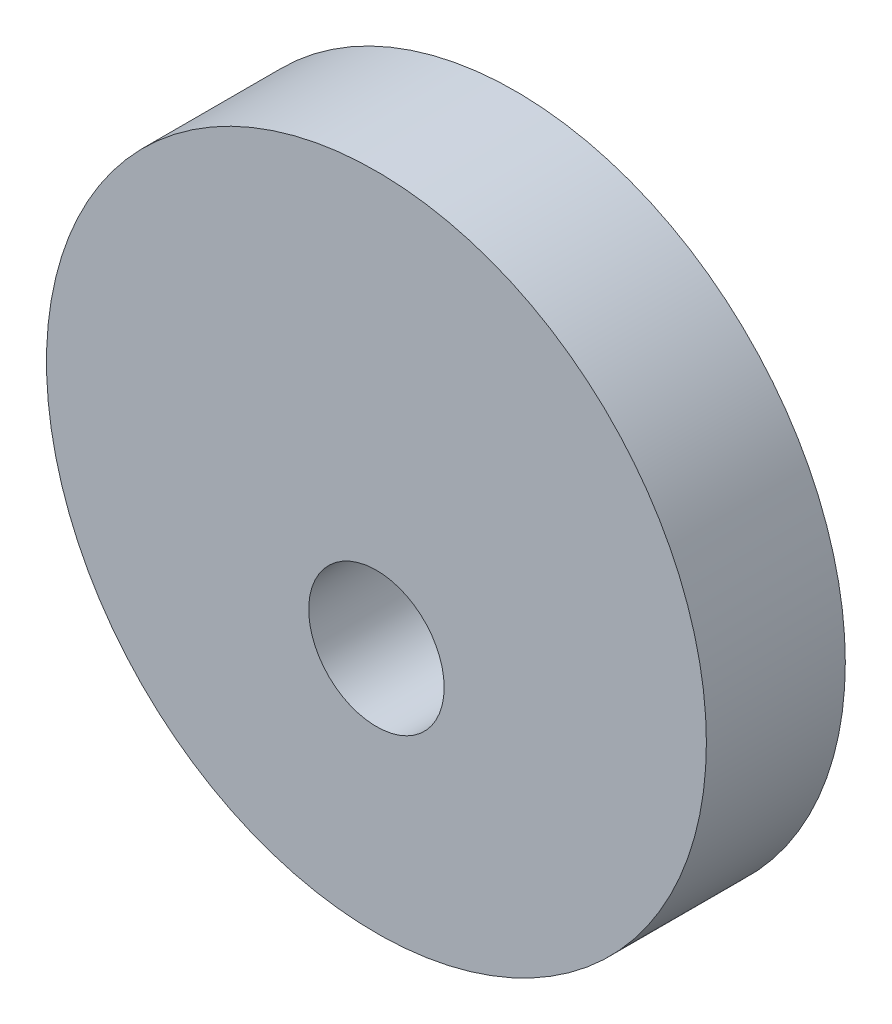
from build123d import *

# Parameters (mm, degrees)
SKETCH1_R           = 19
SKETCH1_R_2         = 3.9
BOSS_EXTRUDE1_DEPTH = 4


with BuildPart() as part:
    # Sketch1 → Boss-Extrude1 (new, symmetric)
    with BuildSketch(Plane.XY):
        with Locations((0, -69.97)):
            Circle(SKETCH1_R)
        with Locations((0, -74.77)):
            Circle(SKETCH1_R_2, mode=Mode.SUBTRACT)
    extrude(amount=BOSS_EXTRUDE1_DEPTH, both=True)


solid = part.part
